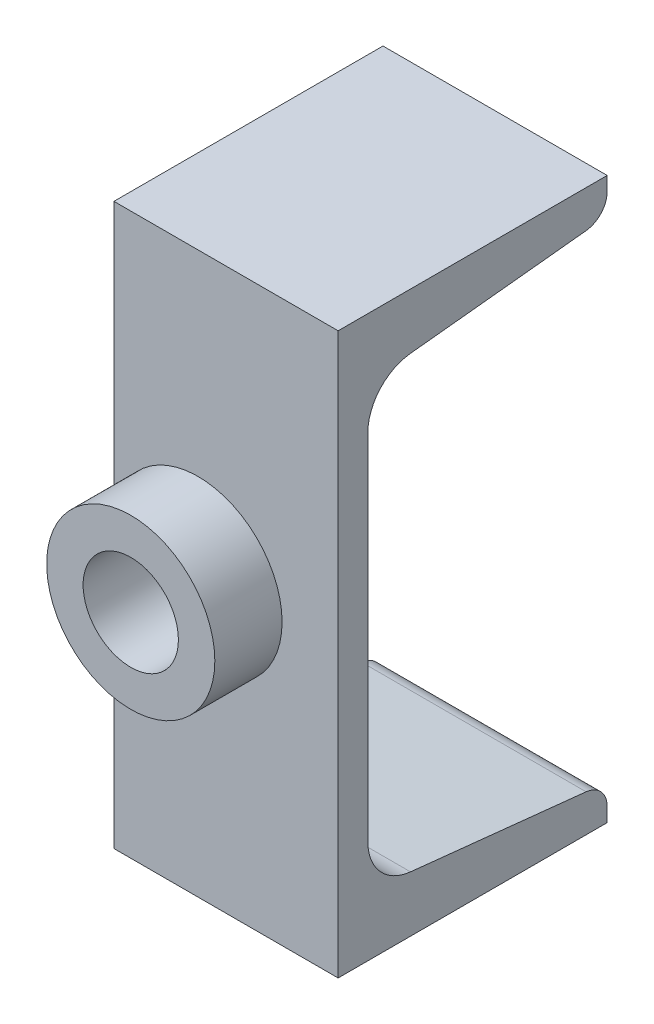
SolidWorks part; units mm, degrees
material "普通碳钢"
ref_plane "Front Plane" through (0, 0, 0) normal (0, 0, 1) x (1, 0, 0)
ref_plane "Top Plane" through (0, 0, 0) normal (0, 1, 0) x (1, 0, 0)
ref_plane "Right Plane" through (0, 0, 0) normal (1, 0, 0) x (0, 0, -1)
sketch3d "3DSketch1"
  line L0 (0, 0, 0) -> (40, 0, 0)
  dimension "D1" = 40
other "Hot-rolled channel gb∕t706-2008 10(1)"
ref_plane "Plane1" through (0, 0, 0) normal (1, 0, 0) x (0, 0, -1)
sketch "Sketch1" plane through (0, 0, 0) normal (1, 0, 0) x (0, 0, -1)
  line L0 (48, 100) -> (0, 100)
  line L1 (48, 0) -> (0, 0)
  line L2 (0, 100) -> (0, 0)
  line L3 (-9.5694, 50) -> (49.7414, 50) construction
  line L4 (5.3, 81.6026) -> (5.3, 18.3974)
  line L5 (48, 0) -> (48, 2.4743)
  line L6 (48, 100) -> (48, 97.5257)
  line L7 (12.9115, 9.944) -> (44.239, 6.6513)
  line L17 (12.9115, 90.056) -> (44.239, 93.3487)
  arc A0 (44.239, 93.3487) -> (48, 97.5257) centre (43.8, 97.5257) ccw
  arc A1 (44.239, 6.6513) -> (48, 2.4743) centre (43.8, 2.4743) cw
  arc A2 (5.3, 18.3974) -> (12.9115, 9.944) centre (13.8, 18.3974) ccw
  arc A10 (5.3, 81.6026) -> (12.9115, 90.056) centre (13.8, 81.6026) cw
  point P6 (0, 0)
  point P8 (0, 50)
  point P9 (5.3, 25.8841)
  point P10 (24, 100)
  point P13 (48, 93.744)
  point P14 (26.65, 91.5)
  point P19 (5.3, 50)
sketch "Sketch2" plane through (0, 0, 0) normal (0, 0, 1) x (1, 0, 0)
  line L0 (0, 50) -> (15, 50) construction
  line L1 (0, 100) -> (0, 0) construction
  line L2 (15, 50) -> (15, 100) construction
  circle A0 centre (15, 50) radius 8.5
  dimension "D1" = 17
  dimension "D2" = 15
extrude "Cut-Extrude1" cut sketch "Sketch2" against normal blind 10
sketch "Sketch3" plane through (0, 0, 0) normal (0, 0, 1) x (1, 0, 0)
  circle A0 centre (15, 50) radius 15
  circle A1 centre (15, 50) radius 8.5
  dimension "D1" = 30
extrude "Boss-Extrude1" add sketch "Sketch3" along normal blind 12 separate body
equation "\"RI@Sketch1\" = \"D1@Sketch1\""
equation "\"D3@Sketch1\" =  ( \"BF@Sketch1\" - \"D6@Sketch1\" )  / 2"
